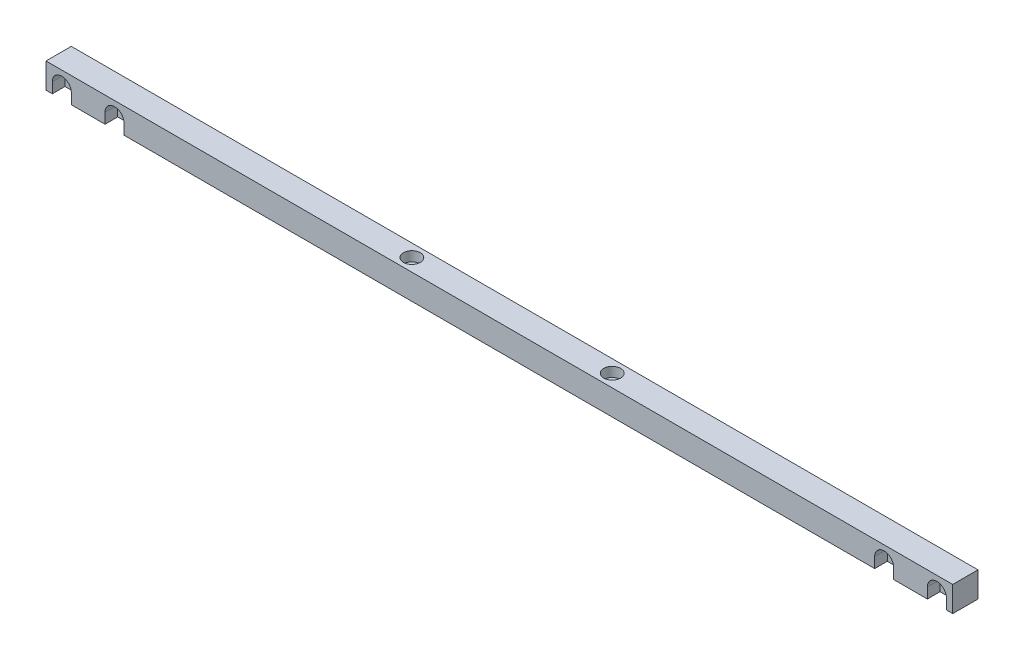
from build123d import *

# Parameters (mm, degrees)
SKETCH_1_W                = 430
SKETCH_1_H                = 12
EXTRUDE_1_DEPTH           = 6
HOLE_WIZARD_5_5_5_5_1_D   = 5.5
HOLE_WIZARD_2_D           = 4.5
HOLE_WIZARD_2_DEPTH       = 14
HOLE_WIZARD_2_CBORE_D     = 8
HOLE_WIZARD_2_CBORE_DEPTH = 4.6
HOLE_WIZARD_2_TIP         = 1.351936393
CUT_EXTRUDE_1_DEPTH       = 6


with BuildPart() as part:
    # 草图1 → 凸台-拉伸1 (new, symmetric)
    with BuildSketch(Plane.XY):
        Rectangle(SKETCH_1_W, SKETCH_1_H)
    extrude(amount=EXTRUDE_1_DEPTH, both=True)

    # Ø5.5 (5.5) 直径孔1 (through all)
    with Locations(Plane.XY.offset(6)):
        with Locations((-207.5, -1), (-182.5, -1), (182.5, -1), (207.5, -1)):
            Hole(HOLE_WIZARD_5_5_5_5_1_D / 2)

    # 打孔尺寸(%根据)内六角圆柱头螺钉的类型2
    with Locations(Plane(origin=(0, 6, 0), x_dir=(1, 0, 0), z_dir=(0, 1, 0))):
        with Locations((-47.5, 0), (47.5, 0)):
            CounterBoreHole(HOLE_WIZARD_2_D / 2, HOLE_WIZARD_2_CBORE_D / 2, HOLE_WIZARD_2_CBORE_DEPTH, depth=HOLE_WIZARD_2_DEPTH)
            with Locations((0, 0, -(HOLE_WIZARD_2_DEPTH + HOLE_WIZARD_2_TIP / 2))):  # 118° drill point
                Cone(0, HOLE_WIZARD_2_D / 2, HOLE_WIZARD_2_TIP, mode=Mode.SUBTRACT)

    # 草图9 → 切除-拉伸1 (cut)
    with BuildSketch(Plane.XY.offset(6)):
        with BuildLine():
            Line((-203, -1), (-203, -15.234595698))
            ThreePointArc((-203, -15.234595698), (-207.5, -19.734595698), (-212, -15.234595698))
            Line((-212, -15.234595698), (-212, -1))
            ThreePointArc((-212, -1), (-207.5, 3.5), (-203, -1))
        make_face()
        with BuildLine():
            Line((-178, -1), (-178, -15.234595698))
            ThreePointArc((-178, -15.234595698), (-182.5, -19.734595698), (-187, -15.234595698))
            Line((-187, -15.234595698), (-187, -1))
            ThreePointArc((-187, -1), (-182.5, 3.5), (-178, -1))
        make_face()
        with BuildLine():
            Line((187, -1), (187, -15.234595698))
            ThreePointArc((187, -15.234595698), (182.5, -19.734595698), (178, -15.234595698))
            Line((178, -15.234595698), (178, -1))
            ThreePointArc((178, -1), (182.5, 3.5), (187, -1))
        make_face()
        with BuildLine():
            Line((212, -1), (212, -15.234595698))
            ThreePointArc((212, -15.234595698), (207.5, -19.734595698), (203, -15.234595698))
            Line((203, -15.234595698), (203, -1))
            ThreePointArc((203, -1), (207.5, 3.5), (212, -1))
        make_face()
    extrude(amount=-CUT_EXTRUDE_1_DEPTH, mode=Mode.SUBTRACT)


solid = part.part
